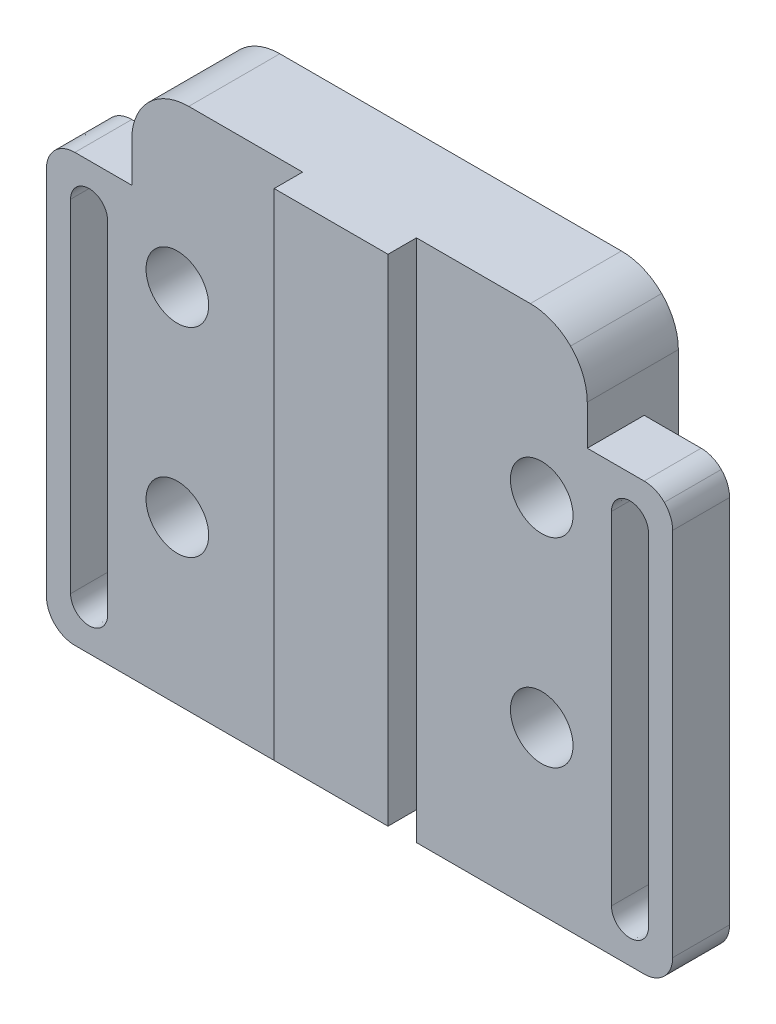
SolidWorks part; units mm, degrees
ref_plane "Front Plane" through (0, 0, 0) normal (0, 0, 1) x (1, 0, 0)
ref_plane "Top Plane" through (0, 0, 0) normal (0, 1, 0) x (1, 0, 0)
ref_plane "Right Plane" through (0, 0, 0) normal (1, 0, 0) x (0, 0, -1)
sketch "Sketch1" plane through (0, 0, 0) normal (0, 0, 1) x (1, 0, 0)
  line L0 (46.2506, -79.8718) -> (46.2506, -72.8718)
  line L1 (-43.7494, -154.8718) -> (56.2506, -154.8718)
  line L2 (-33.7494, -79.8718) -> (-33.7494, -72.8718)
  line L3 (36.2506, -62.8718) -> (-23.7494, -62.8718)
  line L4 (-48.7494, -84.8718) -> (-48.7494, -149.8718)
  line L5 (-33.7494, -79.8718) -> (-43.7494, -79.8718)
  line L6 (-37.9994, -87.3718) -> (-37.9994, -147.3718)
  line L7 (-44.4994, -147.3718) -> (-44.4994, -87.3718)
  line L8 (56.2506, -79.8718) -> (46.2506, -79.8718)
  line L9 (57.0006, -87.3718) -> (57.0006, -147.3718)
  line L10 (50.5006, -147.3718) -> (50.5006, -87.3718)
  line L11 (61.2506, -149.8718) -> (61.2506, -84.8718)
  spline S0 degree 3 poles (43.3217, -65.8007) (43.2437, -65.7242) (43.0879, -65.5713) (42.8451, -65.3519) (42.5959, -65.1403) (42.3398, -64.9371) (42.0768, -64.7421) (41.6283, -64.4317) (40.9724, -64.0382) (40.0838, -63.6184) (39.1583, -63.2868) (38.3634, -63.0881) (37.7184, -62.9759) (37.2313, -62.9161) (36.7418, -62.8787) (36.4145, -62.8741) (36.2506, -62.8718) knots 0 0 0 0 0.041739 0.083393 0.125006 0.166623 0.208289 0.250048 0.374992 0.500007 0.624951 0.749966 0.812537 0.874965 0.937403 1 1 1 1
  spline S1 degree 3 poles (46.2506, -72.8718) (46.2496, -72.7626) (46.2476, -72.5443) (46.231, -72.2174) (46.2044, -71.8916) (46.167, -71.5668) (46.1189, -71.243) (46.0213, -70.7063) (45.8357, -69.9643) (45.5043, -69.0391) (45.0843, -68.1503) (44.6627, -67.4476) (44.286, -66.9122) (43.9838, -66.5255) (43.6641, -66.1529) (43.436, -65.9182) (43.3217, -65.8007) knots 0 0 0 0 0.041739 0.083393 0.125006 0.166623 0.208289 0.250048 0.374992 0.500007 0.624951 0.749966 0.812537 0.874965 0.937403 1 1 1 1
  spline S2 degree 3 poles (-30.8204, -65.8007) (-30.897, -65.8787) (-31.0499, -66.0345) (-31.2692, -66.2774) (-31.4809, -66.5266) (-31.6841, -66.7827) (-31.879, -67.0456) (-32.1894, -67.4942) (-32.5829, -68.1501) (-33.0028, -69.0387) (-33.3344, -69.9641) (-33.5331, -70.7591) (-33.6453, -71.404) (-33.705, -71.8911) (-33.7424, -72.3807) (-33.747, -72.708) (-33.7494, -72.8718) knots 0 0 0 0 0.041739 0.083393 0.125006 0.166623 0.208289 0.250048 0.374992 0.500007 0.624951 0.749966 0.812537 0.874965 0.937403 1 1 1 1
  spline S3 degree 3 poles (-23.7494, -62.8718) (-23.8586, -62.8728) (-24.0769, -62.8749) (-24.4037, -62.8915) (-24.7296, -62.918) (-25.0544, -62.9555) (-25.3782, -63.0035) (-25.9148, -63.1012) (-26.6569, -63.2868) (-27.5821, -63.6182) (-28.4709, -64.0381) (-29.1736, -64.4597) (-29.7089, -64.8365) (-30.0956, -65.1386) (-30.4682, -65.4583) (-30.7029, -65.6865) (-30.8204, -65.8007) knots 0 0 0 0 0.041739 0.083393 0.125006 0.166623 0.208289 0.250048 0.374992 0.500007 0.624951 0.749966 0.812537 0.874965 0.937403 1 1 1 1
  spline S4 degree 3 poles (-25.7494, -94.6218) (-25.6881, -94.6209) (-25.5661, -94.6189) (-25.3842, -94.6032) (-25.2042, -94.5781) (-25.0263, -94.5427) (-24.8503, -94.4972) (-24.6763, -94.4415) (-24.3639, -94.3221) (-23.9314, -94.0925) (-23.437, -93.6845) (-23.0287, -93.1898) (-22.728, -92.6235) (-22.5401, -92.0103) (-22.479, -91.372) (-22.54, -90.7335) (-22.7279, -90.1205) (-23.0286, -89.554) (-23.4368, -89.0595) (-23.9313, -88.6512) (-24.4042, -88.4003) (-24.8047, -88.2562) (-25.114, -88.1788) (-25.4296, -88.1306) (-25.6424, -88.1248) (-25.7494, -88.1218) knots 0 0 0 0 0.018013 0.035886 0.053676 0.07144 0.089234 0.107116 0.125143 0.187594 0.2501 0.312552 0.375058 0.43751 0.500016 0.562468 0.624974 0.687426 0.749932 0.812384 0.87489 0.90631 0.937431 0.968559 1 1 1 1
  spline S5 degree 3 poles (-25.7494, -88.1218) (-25.8106, -88.1228) (-25.9326, -88.1247) (-26.1145, -88.1404) (-26.2945, -88.1655) (-26.4724, -88.201) (-26.6484, -88.2465) (-26.8224, -88.3021) (-27.1348, -88.4216) (-27.5673, -88.6511) (-28.0617, -89.0592) (-28.47, -89.5538) (-28.7707, -90.1201) (-28.9586, -90.7334) (-29.0197, -91.3716) (-28.9587, -92.0101) (-28.7708, -92.6232) (-28.4701, -93.1896) (-28.0619, -93.6842) (-27.5674, -94.0925) (-27.0945, -94.3433) (-26.694, -94.4875) (-26.3847, -94.5648) (-26.0691, -94.613) (-25.8563, -94.6189) (-25.7494, -94.6218) knots 0 0 0 0 0.018013 0.035886 0.053676 0.07144 0.089234 0.107116 0.125143 0.187594 0.2501 0.312552 0.375058 0.43751 0.500016 0.562468 0.624974 0.687426 0.749932 0.812384 0.87489 0.90631 0.937431 0.968559 1 1 1 1
  spline S6 degree 3 poles (-25.7494, -123.1218) (-25.3239, -123.1218) (-24.8987, -123.2064) (-24.1126, -123.532) (-23.7521, -123.7729) (-23.1504, -124.3745) (-22.9095, -124.7351) (-22.5839, -125.5211) (-22.4994, -125.9464) (-22.4994, -126.7972) (-22.5839, -127.2225) (-22.9095, -128.0086) (-23.1504, -128.3691) (-23.7521, -128.9707) (-24.1126, -129.2116) (-24.8987, -129.5372) (-25.3239, -129.6218) (-25.7494, -129.6218) knots 0 0 0 0 0.125 0.125 0.25 0.25 0.375 0.375 0.5 0.5 0.625 0.625 0.75 0.75 0.875 0.875 1 1 1 1
  spline S7 degree 3 poles (-25.7494, -129.6218) (-26.1748, -129.6218) (-26.6, -129.5372) (-27.3861, -129.2116) (-27.7466, -128.9707) (-28.3483, -128.3691) (-28.5892, -128.0086) (-28.9148, -127.2225) (-28.9994, -126.7972) (-28.9994, -125.9464) (-28.9148, -125.5211) (-28.5892, -124.7351) (-28.3483, -124.3745) (-27.7466, -123.7729) (-27.3861, -123.532) (-26.6, -123.2064) (-26.1748, -123.1218) (-25.7494, -123.1218) knots 0 0 0 0 0.125 0.125 0.25 0.25 0.375 0.375 0.5 0.5 0.625 0.625 0.75 0.75 0.875 0.875 1 1 1 1
  spline S8 degree 3 poles (38.2506, -129.6218) (37.8252, -129.6218) (37.4, -129.5372) (36.6139, -129.2116) (36.2534, -128.9707) (35.6517, -128.3691) (35.4108, -128.0086) (35.0852, -127.2225) (35.0006, -126.7972) (35.0006, -125.9464) (35.0852, -125.5211) (35.4108, -124.7351) (35.6517, -124.3745) (36.2534, -123.7729) (36.6139, -123.532) (37.4, -123.2064) (37.8252, -123.1218) (38.2506, -123.1218) knots 0 0 0 0 0.125 0.125 0.25 0.25 0.375 0.375 0.5 0.5 0.625 0.625 0.75 0.75 0.875 0.875 1 1 1 1
  spline S9 degree 3 poles (38.2506, -88.1218) (38.6761, -88.1218) (39.1013, -88.2064) (39.8874, -88.532) (40.2479, -88.7729) (40.8496, -89.3745) (41.0905, -89.7351) (41.4161, -90.5211) (41.5006, -90.9464) (41.5006, -91.7972) (41.4161, -92.2225) (41.0905, -93.0086) (40.8496, -93.3691) (40.2479, -93.9707) (39.8874, -94.2116) (39.1013, -94.5372) (38.6761, -94.6218) (38.2506, -94.6218) knots 0 0 0 0 0.125 0.125 0.25 0.25 0.375 0.375 0.5 0.5 0.625 0.625 0.75 0.75 0.875 0.875 1 1 1 1
  spline S10 degree 3 poles (38.2506, -94.6218) (37.8252, -94.6218) (37.4, -94.5372) (36.6139, -94.2116) (36.2534, -93.9707) (35.6517, -93.3691) (35.4108, -93.0086) (35.0852, -92.2225) (35.0006, -91.7972) (35.0006, -90.9464) (35.0852, -90.5211) (35.4108, -89.7351) (35.6517, -89.3745) (36.2534, -88.7729) (36.6139, -88.532) (37.4, -88.2064) (37.8252, -88.1218) (38.2506, -88.1218) knots 0 0 0 0 0.125 0.125 0.25 0.25 0.375 0.375 0.5 0.5 0.625 0.625 0.75 0.75 0.875 0.875 1 1 1 1
  spline S11 degree 3 poles (38.2506, -123.1218) (38.6761, -123.1218) (39.1013, -123.2064) (39.8874, -123.532) (40.2479, -123.7729) (40.8496, -124.3745) (41.0905, -124.7351) (41.4161, -125.5211) (41.5006, -125.9464) (41.5006, -126.7972) (41.4161, -127.2225) (41.0905, -128.0086) (40.8496, -128.3691) (40.2479, -128.9707) (39.8874, -129.2116) (39.1013, -129.5372) (38.6761, -129.6218) (38.2506, -129.6218) knots 0 0 0 0 0.125 0.125 0.25 0.25 0.375 0.375 0.5 0.5 0.625 0.625 0.75 0.75 0.875 0.875 1 1 1 1
  spline S12 degree 3 poles (-47.2849, -153.4073) (-47.238, -153.4532) (-47.1444, -153.5447) (-46.9974, -153.6748) (-46.8458, -153.7993) (-46.6892, -153.9178) (-46.4476, -154.0862) (-46.1102, -154.2886) (-45.666, -154.4985) (-45.2032, -154.6643) (-44.7793, -154.7704) (-44.4025, -154.8324) (-44.0767, -154.8657) (-43.8586, -154.8698) (-43.7494, -154.8718) knots 0 0 0 0 0.050065 0.100025 0.149957 0.199939 0.250049 0.374961 0.500014 0.624926 0.749979 0.833348 0.916569 1 1 1 1
  spline S13 degree 3 poles (-48.7494, -149.8718) (-48.7486, -149.9373) (-48.7471, -150.0682) (-48.7352, -150.2642) (-48.7161, -150.4594) (-48.6891, -150.654) (-48.6373, -150.9439) (-48.5419, -151.3255) (-48.3762, -151.7881) (-48.1662, -152.2325) (-47.9415, -152.6073) (-47.7189, -152.9176) (-47.512, -153.1716) (-47.3607, -153.3287) (-47.2849, -153.4073) knots 0 0 0 0 0.050065 0.100025 0.149957 0.199939 0.250049 0.374961 0.500014 0.624926 0.749979 0.833348 0.916569 1 1 1 1
  spline S14 degree 3 poles (-47.2849, -81.3363) (-47.3307, -81.3831) (-47.4222, -81.4767) (-47.5523, -81.6238) (-47.6769, -81.7753) (-47.7953, -81.932) (-47.9637, -82.1736) (-48.1661, -82.5109) (-48.3761, -82.9552) (-48.5418, -83.4179) (-48.648, -83.8418) (-48.7099, -84.2186) (-48.7432, -84.5445) (-48.7473, -84.7626) (-48.7494, -84.8718) knots 0 0 0 0 0.050065 0.100025 0.149957 0.199939 0.250049 0.374961 0.500014 0.624926 0.749979 0.833348 0.916569 1 1 1 1
  spline S15 degree 3 poles (-43.7494, -79.8718) (-43.8149, -79.8726) (-43.9458, -79.874) (-44.1417, -79.886) (-44.337, -79.9051) (-44.5315, -79.9321) (-44.8214, -79.9838) (-45.2031, -80.0793) (-45.6657, -80.245) (-46.1101, -80.455) (-46.4849, -80.6797) (-46.7951, -80.9023) (-47.0491, -81.1092) (-47.2062, -81.2605) (-47.2849, -81.3363) knots 0 0 0 0 0.050065 0.100025 0.149957 0.199939 0.250049 0.374961 0.500014 0.624926 0.749979 0.833348 0.916569 1 1 1 1
  spline S16 degree 3 poles (-38.9513, -149.6699) (-38.9895, -149.7071) (-39.0659, -149.7814) (-39.1869, -149.8853) (-39.3123, -149.9834) (-39.4425, -150.075) (-39.5774, -150.1604) (-39.8088, -150.2914) (-40.1503, -150.4433) (-40.6128, -150.5707) (-41.0893, -150.63) (-41.7277, -150.6139) (-42.5113, -150.4185) (-43.2035, -150.0027) (-43.6663, -149.5626) (-43.9612, -149.184) (-44.1982, -148.7667) (-44.3515, -148.3682) (-44.4419, -148.007) (-44.4905, -147.691) (-44.4964, -147.4784) (-44.4994, -147.3718) knots 0 0 0 0 0.020935 0.041773 0.062565 0.08336 0.10421 0.125165 0.187662 0.250231 0.312727 0.375296 0.500018 0.624741 0.687237 0.749806 0.812302 0.874871 0.916632 0.958207 1 1 1 1
  spline S17 degree 3 poles (-37.9994, -147.3718) (-38.0003, -147.4331) (-38.0022, -147.5551) (-38.0179, -147.737) (-38.0431, -147.9169) (-38.0785, -148.0949) (-38.124, -148.2709) (-38.1797, -148.4448) (-38.2615, -148.6587) (-38.3783, -148.907) (-38.5423, -149.1804) (-38.7314, -149.4376) (-38.8777, -149.5922) (-38.9513, -149.6699) knots 0 0 0 0 0.071979 0.1434 0.214488 0.28547 0.356576 0.428033 0.500065 0.625619 0.749978 0.874364 1 1 1 1
  spline S18 degree 3 poles (-38.9513, -85.0737) (-38.9086, -85.1177) (-38.8237, -85.2053) (-38.7062, -85.3451) (-38.5967, -85.4901) (-38.4959, -85.641) (-38.4037, -85.7976) (-38.32, -85.96) (-38.2266, -86.169) (-38.1337, -86.4272) (-38.0564, -86.7365) (-38.0081, -87.0521) (-38.0023, -87.2649) (-37.9994, -87.3718) knots 0 0 0 0 0.071979 0.1434 0.214488 0.28547 0.356576 0.428033 0.500065 0.625619 0.749978 0.874364 1 1 1 1
  spline S19 degree 3 poles (-44.4994, -87.3718) (-44.4986, -87.3184) (-44.4971, -87.212) (-44.485, -87.0528) (-44.4657, -86.8949) (-44.4384, -86.738) (-44.4034, -86.5822) (-44.3324, -86.326) (-44.1983, -85.9771) (-43.9614, -85.5599) (-43.6664, -85.1812) (-43.2036, -84.7411) (-42.5113, -84.3251) (-41.7279, -84.1298) (-41.0894, -84.1136) (-40.6132, -84.1729) (-40.1505, -84.3003) (-39.7603, -84.4737) (-39.4411, -84.6652) (-39.1832, -84.8543) (-39.0287, -85.0005) (-38.9513, -85.0737) knots 0 0 0 0 0.020935 0.041773 0.062565 0.08336 0.10421 0.125165 0.187662 0.250231 0.312727 0.375296 0.500018 0.624741 0.687237 0.749806 0.812302 0.874871 0.916632 0.958207 1 1 1 1
  spline S20 degree 3 poles (59.7862, -81.3363) (59.7393, -81.2905) (59.6457, -81.1989) (59.4987, -81.0688) (59.3471, -80.9443) (59.1905, -80.8258) (58.9489, -80.6574) (58.6115, -80.4551) (58.1673, -80.2451) (57.7045, -80.0794) (57.2806, -79.9732) (56.9038, -79.9112) (56.578, -79.8779) (56.3598, -79.8739) (56.2506, -79.8718) knots 0 0 0 0 0.050065 0.100025 0.149957 0.199939 0.250049 0.374961 0.500014 0.624926 0.749979 0.833348 0.916569 1 1 1 1
  spline S21 degree 3 poles (61.2506, -84.8718) (61.2499, -84.8063) (61.2484, -84.6754) (61.2365, -84.4794) (61.2174, -84.2842) (61.1904, -84.0897) (61.1386, -83.7997) (61.0432, -83.4181) (60.8775, -82.9555) (60.6675, -82.5111) (60.4428, -82.1363) (60.2202, -81.826) (60.0133, -81.5721) (59.862, -81.4149) (59.7862, -81.3363) knots 0 0 0 0 0.050065 0.100025 0.149957 0.199939 0.250049 0.374961 0.500014 0.624926 0.749979 0.833348 0.916569 1 1 1 1
  spline S22 degree 3 poles (56.0487, -85.0737) (56.0914, -85.1177) (56.1763, -85.2053) (56.2938, -85.3451) (56.4033, -85.4901) (56.5041, -85.641) (56.5963, -85.7976) (56.68, -85.96) (56.7734, -86.169) (56.8663, -86.4272) (56.9436, -86.7365) (56.9919, -87.0521) (56.9977, -87.2649) (57.0006, -87.3718) knots 0 0 0 0 0.071979 0.1434 0.214488 0.28547 0.356576 0.428033 0.500065 0.625619 0.749978 0.874364 1 1 1 1
  spline S23 degree 3 poles (50.5006, -87.3718) (50.5014, -87.3184) (50.5029, -87.212) (50.515, -87.0528) (50.5343, -86.8949) (50.5616, -86.738) (50.5966, -86.5822) (50.6676, -86.326) (50.8017, -85.9771) (51.0386, -85.5599) (51.3336, -85.1812) (51.7964, -84.7411) (52.4887, -84.3251) (53.2721, -84.1298) (53.9106, -84.1136) (54.3868, -84.1729) (54.8495, -84.3003) (55.2397, -84.4737) (55.5589, -84.6652) (55.8168, -84.8543) (55.9713, -85.0005) (56.0487, -85.0737) knots 0 0 0 0 0.020935 0.041773 0.062565 0.08336 0.10421 0.125165 0.187662 0.250231 0.312727 0.375296 0.500018 0.624741 0.687237 0.749806 0.812302 0.874871 0.916632 0.958207 1 1 1 1
  spline S24 degree 3 poles (57.0006, -147.3718) (56.9997, -147.4331) (56.9978, -147.5551) (56.9821, -147.737) (56.9569, -147.9169) (56.9215, -148.0949) (56.876, -148.2709) (56.8203, -148.4448) (56.7385, -148.6587) (56.6217, -148.907) (56.4577, -149.1804) (56.2686, -149.4376) (56.1223, -149.5922) (56.0487, -149.6699) knots 0 0 0 0 0.071979 0.1434 0.214488 0.28547 0.356576 0.428033 0.500065 0.625619 0.749978 0.874364 1 1 1 1
  spline S25 degree 3 poles (59.7862, -153.4073) (59.832, -153.3605) (59.9235, -153.2669) (60.0536, -153.1199) (60.1782, -152.9683) (60.2966, -152.8117) (60.465, -152.5701) (60.6674, -152.2327) (60.8774, -151.7885) (61.0431, -151.3257) (61.1492, -150.9018) (61.2112, -150.525) (61.2445, -150.1991) (61.2486, -149.981) (61.2506, -149.8718) knots 0 0 0 0 0.050065 0.100025 0.149957 0.199939 0.250049 0.374961 0.500014 0.624926 0.749979 0.833348 0.916569 1 1 1 1
  spline S26 degree 3 poles (56.0487, -149.6699) (56.0105, -149.7071) (55.9341, -149.7814) (55.8131, -149.8853) (55.6877, -149.9834) (55.5575, -150.075) (55.4226, -150.1604) (55.1912, -150.2914) (54.8497, -150.4433) (54.3872, -150.5707) (53.9107, -150.63) (53.2723, -150.6139) (52.4887, -150.4185) (51.7965, -150.0027) (51.3337, -149.5626) (51.0388, -149.184) (50.8018, -148.7667) (50.6485, -148.3682) (50.5581, -148.007) (50.5095, -147.691) (50.5036, -147.4784) (50.5006, -147.3718) knots 0 0 0 0 0.020935 0.041773 0.062565 0.08336 0.10421 0.125165 0.187662 0.250231 0.312727 0.375296 0.500018 0.624741 0.687237 0.749806 0.812302 0.874871 0.916632 0.958207 1 1 1 1
  spline S27 degree 3 poles (56.2506, -154.8718) (56.3162, -154.8711) (56.4471, -154.8696) (56.643, -154.8576) (56.8383, -154.8385) (57.0328, -154.8116) (57.3227, -154.7598) (57.7044, -154.6643) (58.167, -154.4987) (58.6114, -154.2886) (58.9862, -154.064) (59.2964, -153.8414) (59.5504, -153.6345) (59.7075, -153.4831) (59.7862, -153.4073) knots 0 0 0 0 0.050065 0.100025 0.149957 0.199939 0.250049 0.374961 0.500014 0.624926 0.749979 0.833348 0.916569 1 1 1 1
extrude "Boss-Extrude1" add sketch "Sketch1" along normal blind 16
sketch "Sketch2" plane through (0, 0, 16) normal (0, 0, 1) x (1, 0, 0)
  line L0 (36.2506, -62.8718) -> (-23.7494, -62.8718) construction
  line L1 (16.2506, -149.8718) -> (-3.7494, -149.8718)
  line L2 (16.2506, -149.8718) -> (16.2506, -62.8718)
  line L3 (16.2506, -62.8718) -> (-3.7494, -62.8718)
  line L4 (-3.7494, -149.8718) -> (-3.7494, -62.8718)
  line L5 (16.2506, -149.8718) -> (-3.7494, -62.8718) construction
  line L6 (16.2506, -62.8718) -> (-3.7494, -149.8718) construction
  line L7 (-43.7494, -154.8718) -> (56.2506, -154.8718) construction
  point P0 (6.2506, -106.3718)
  point P9 (6.2506, -62.8718)
  point P13 (6.2506, -154.8718)
  dimension "D1" = 20
  dimension "D2" = 87
extrude "Boss-Extrude2" add sketch "Sketch2" along normal blind 5
sketch "Sketch3" plane through (0, 0, 21) normal (0, 0, 1) x (1, 0, 0)
  line L0 (-3.7494, -149.8718) -> (-3.7494, -154.8718)
  line L1 (-43.7494, -154.8718) -> (56.2506, -154.8718) construction
  line L2 (-3.7494, -154.8718) -> (16.2506, -154.8718)
  line L3 (16.2506, -154.8718) -> (16.2506, -149.8718)
  line L4 (16.2506, -149.8718) -> (-3.7494, -149.8718)
extrude "Cut-Extrude1" cut sketch "Sketch3" against normal blind 11
sketch "Sketch4" plane through (0, 0, 16) normal (0, 0, 1) x (1, 0, 0)
  line L3 (-25.7494, -126.3718) -> (-16.5569, -126.3718) construction
  circle A0 centre (-25.7494, -126.3718) radius 5.5
  circle A1 centre (38.2506, -126.3718) radius 5.5
  circle A2 centre (38.2506, -91.3718) radius 5.5
  circle A3 centre (-25.7494, -91.3718) radius 5.5
  dimension "D1" = 11
  dimension "D2" = 2
  dimension "D3" = 2
extrude "Cut-Extrude2" cut sketch "Sketch4" against normal blind 10
sketch "Sketch5" plane through (0, 0, 0) normal (0, 0, -1) x (-1, 0, 0)
  line L1 (-30.2506, -131.3718) -> (-46.2506, -131.3718)
  line L2 (-30.2506, -131.3718) -> (-30.2506, -86.3718)
  line L3 (-30.2506, -86.3718) -> (-46.2506, -86.3718)
  line L4 (-46.2506, -131.3718) -> (-46.2506, -86.3718)
  line L5 (-30.2506, -131.3718) -> (-46.2506, -86.3718) construction
  line L6 (-30.2506, -86.3718) -> (-46.2506, -131.3718) construction
  line L9 (-46.2506, -79.8718) -> (-46.2506, -72.8718) construction
  line L10 (-6.2506, -62.8718) -> (-6.2506, -73.4746) construction
  line L11 (-36.2506, -62.8718) -> (23.7494, -62.8718) construction
  line L12 (17.7494, -86.3718) -> (33.7494, -131.3718) construction
  line L13 (17.7494, -131.3718) -> (33.7494, -86.3718) construction
  line L16 (33.7494, -131.3718) -> (33.7494, -86.3718)
  line L17 (17.7494, -86.3718) -> (33.7494, -86.3718)
  line L18 (17.7494, -131.3718) -> (17.7494, -86.3718)
  line L19 (17.7494, -131.3718) -> (33.7494, -131.3718)
  point P0 (-38.2506, -108.8718)
  point P25 (25.7494, -108.8718)
  dimension "D1" = 16
  dimension "D2" = 45
extrude "Cut-Extrude3" cut sketch "Sketch5" against normal blind 1
sketch "Sketch6" plane through (0, 0, 0) normal (0, 0, -1) x (-1, 0, 0)
  line L0 (-46.2506, -79.8718) -> (-46.2506, -154.8718)
  line L1 (43.7494, -154.8718) -> (-56.2506, -154.8718) construction
  line L2 (-57.0006, -147.3718) -> (-57.0006, -87.3718) construction
  line L3 (-57.0006, -147.3718) -> (-57.0006, -87.3718)
  line L4 (-50.5006, -87.3718) -> (-50.5006, -147.3718) construction
  line L5 (-50.5006, -87.3718) -> (-50.5006, -147.3718)
  line L6 (-46.2506, -154.8718) -> (-56.2506, -154.8718)
  line L7 (-6.2506, -154.8718) -> (-6.2506, -140.574) construction
  line L10 (-46.2506, -72.8718) -> (-46.2506, -79.8718)
  line L11 (-46.2506, -79.8718) -> (-56.2506, -79.8718)
  line L12 (-61.2506, -84.8718) -> (-61.2506, -149.8718)
  line L13 (-56.2506, -154.8718) -> (43.7494, -154.8718)
  line L14 (48.7494, -149.8718) -> (48.7494, -84.8718)
  line L15 (43.7494, -79.8718) -> (33.7494, -79.8718)
  line L16 (33.7494, -79.8718) -> (33.7494, -72.8718)
  line L17 (23.7494, -62.8718) -> (-36.2506, -62.8718)
  line L19 (-46.2506, -79.8718) -> (-56.2506, -79.8718)
  line L20 (-61.2506, -84.8718) -> (-61.2506, -149.8718)
  line L30 (33.7494, -79.8718) -> (33.7494, -154.8718)
  line L31 (33.7494, -154.8718) -> (43.7494, -154.8718)
  line L32 (33.7494, -79.8718) -> (43.7494, -79.8718)
  line L33 (48.7494, -84.8718) -> (48.7494, -149.8718) construction
  line L34 (48.7494, -84.8718) -> (48.7494, -149.8718)
  line L35 (44.4994, -87.3718) -> (44.4994, -147.3718) construction
  line L36 (37.9994, -147.3718) -> (37.9994, -87.3718) construction
  line L37 (44.4994, -87.3718) -> (44.4994, -147.3718)
  line L38 (37.9994, -147.3718) -> (37.9994, -87.3718)
  spline S0 degree 3 poles (-2027.4066, 2176.0249) (-42.345, -125.957) (-62.4154, -89.6938) (-55.5589, -84.6652) (-55.2397, -84.4737) (-54.8495, -84.3003) (-54.3868, -84.1729) (-53.9106, -84.1136) (-53.2721, -84.1298) (-52.4887, -84.3251) (-51.7964, -84.7411) (-51.3336, -85.1812) (-51.0386, -85.5599) (-50.8017, -85.9771) (-50.6676, -86.326) (-50.5966, -86.5822) (-50.5616, -86.738) (-50.5343, -86.8949) (-50.515, -87.0528) (-50.0095, -93.701) (-74.9187, -101.2707) (2947.83, 8.0716) knots -3.202284 -3.202284 -3.202284 -3.202284 0.041793 0.083368 0.125129 0.187698 0.250194 0.312763 0.375259 0.499982 0.624704 0.687273 0.749769 0.812338 0.874835 0.89579 0.91664 0.937435 0.958227 0.979065 3.551551 3.551551 3.551551 3.551551 only from (-56.0487, -85.0737) to (-50.5006, -87.3718) construction
  spline S1 degree 3 poles (-56.0487, -85.0737) (-55.9713, -85.0005) (-55.8168, -84.8543) (-55.5589, -84.6652) (-55.2397, -84.4737) (-54.8495, -84.3003) (-54.3868, -84.1729) (-53.9106, -84.1136) (-53.2721, -84.1298) (-52.4887, -84.3251) (-51.7964, -84.7411) (-51.3336, -85.1812) (-51.0386, -85.5599) (-50.8017, -85.9771) (-50.6676, -86.326) (-50.5966, -86.5822) (-50.5616, -86.738) (-50.5343, -86.8949) (-50.515, -87.0528) (-50.5029, -87.212) (-50.5014, -87.3184) (-50.5006, -87.3718) knots 0 0 0 0 0.041793 0.083368 0.125129 0.187698 0.250194 0.312763 0.375259 0.499982 0.624704 0.687273 0.749769 0.812338 0.874835 0.89579 0.91664 0.937435 0.958227 0.979065 1 1 1 1
  spline S2 degree 3 poles (-3049.9078, 116.4435) (-18.3774, -106.6249) (-58.2318, -95.1636) (-56.9436, -86.7365) (-56.8663, -86.4272) (-56.7734, -86.169) (-56.68, -85.96) (-56.5963, -85.7976) (-56.5041, -85.641) (-56.4033, -85.4901) (-56.2938, -85.3451) (-51.7772, -79.9754) (-26.7535, -93.4896) (-2253.3466, 1957.3042) knots -9.622076 -9.622076 -9.622076 -9.622076 0.125636 0.250022 0.374381 0.499935 0.571967 0.643424 0.71453 0.785512 0.8566 0.928021 9.027047 9.027047 9.027047 9.027047 only from (-57.0006, -87.3718) to (-56.0487, -85.0737) construction
  spline S3 degree 3 poles (-57.0006, -87.3718) (-56.9977, -87.2649) (-56.9919, -87.0521) (-56.9436, -86.7365) (-56.8663, -86.4272) (-56.7734, -86.169) (-56.68, -85.96) (-56.5963, -85.7976) (-56.5041, -85.641) (-56.4033, -85.4901) (-56.2938, -85.3451) (-56.1763, -85.2053) (-56.0914, -85.1177) (-56.0487, -85.0737) knots 0 0 0 0 0.125636 0.250022 0.374381 0.499935 0.571967 0.643424 0.71453 0.785512 0.8566 0.928021 1 1 1 1
  spline S4 degree 3 poles (2942.298, -352.2494) (-89.0995, -128.1529) (-49.2656, -139.603) (-50.5581, -148.007) (-50.6485, -148.3682) (-50.8018, -148.7667) (-51.0388, -149.184) (-51.3337, -149.5626) (-51.7965, -150.0027) (-52.4887, -150.4185) (-53.2723, -150.6139) (-53.9107, -150.63) (-54.3872, -150.5707) (-54.8497, -150.4433) (-55.1912, -150.2914) (-55.4226, -150.1604) (-55.5575, -150.075) (-55.6877, -149.9834) (-55.8131, -149.8853) (-60.8715, -145.5418) (-48.6106, -122.5757) (-2108.7, -2337.2985) knots -3.202284 -3.202284 -3.202284 -3.202284 0.041793 0.083368 0.125129 0.187698 0.250194 0.312763 0.375259 0.499982 0.624704 0.687273 0.749769 0.812338 0.874835 0.89579 0.91664 0.937435 0.958227 0.979065 3.551551 3.551551 3.551551 3.551551 only from (-50.5006, -147.3718) to (-56.0487, -149.6699) construction
  spline S5 degree 3 poles (-50.5006, -147.3718) (-50.5036, -147.4784) (-50.5095, -147.691) (-50.5581, -148.007) (-50.6485, -148.3682) (-50.8018, -148.7667) (-51.0388, -149.184) (-51.3337, -149.5626) (-51.7965, -150.0027) (-52.4887, -150.4185) (-53.2723, -150.6139) (-53.9107, -150.63) (-54.3872, -150.5707) (-54.8497, -150.4433) (-55.1912, -150.2914) (-55.4226, -150.1604) (-55.5575, -150.075) (-55.6877, -149.9834) (-55.8131, -149.8853) (-55.9341, -149.7814) (-56.0105, -149.7071) (-56.0487, -149.6699) knots 0 0 0 0 0.041793 0.083368 0.125129 0.187698 0.250194 0.312763 0.375259 0.499982 0.624704 0.687273 0.749769 0.812338 0.874835 0.89579 0.91664 0.937435 0.958227 0.979065 1 1 1 1
  spline S6 degree 3 poles (-2316.4728, -2121.8557) (-15.124, -135.9732) (-51.4096, -156.0501) (-56.4577, -149.1804) (-56.6217, -148.907) (-56.7385, -148.6587) (-56.8203, -148.4448) (-56.876, -148.2709) (-56.9215, -148.0949) (-56.9569, -147.9169) (-56.9821, -147.737) (-57.5853, -140.7463) (-30.3348, -132.6079) (-3054.9041, -256.9167) knots -9.622076 -9.622076 -9.622076 -9.622076 0.125636 0.250022 0.374381 0.499935 0.571967 0.643424 0.71453 0.785512 0.8566 0.928021 9.027047 9.027047 9.027047 9.027047 only from (-56.0487, -149.6699) to (-57.0006, -147.3718) construction
  spline S7 degree 3 poles (-56.0487, -149.6699) (-56.1223, -149.5922) (-56.2686, -149.4376) (-56.4577, -149.1804) (-56.6217, -148.907) (-56.7385, -148.6587) (-56.8203, -148.4448) (-56.876, -148.2709) (-56.9215, -148.0949) (-56.9569, -147.9169) (-56.9821, -147.737) (-56.9978, -147.5551) (-56.9997, -147.4331) (-57.0006, -147.3718) knots 0 0 0 0 0.125636 0.250022 0.374381 0.499935 0.571967 0.643424 0.71453 0.785512 0.8566 0.928021 1 1 1 1
  spline S8 degree 3 poles (2216.2512, 1990.9412) (18.2653, -86.6751) (42.1004, -75.4628) (47.5523, -81.6238) (47.6769, -81.7753) (47.7953, -81.932) (47.9637, -82.1736) (48.1661, -82.5109) (48.3761, -82.9552) (48.5418, -83.4179) (48.648, -83.8418) (48.7099, -84.2186) (49.7106, -94.015) (14.6956, -105.5474) (3046.0394, 40.1273) knots -6.134029 -6.134029 -6.134029 -6.134029 0.050065 0.100025 0.149957 0.199939 0.250049 0.374961 0.500014 0.624926 0.749979 0.833348 0.916569 8.266403 8.266403 8.266403 8.266403 only from (47.2849, -81.3363) to (48.7494, -84.8718) construction
  spline S9 degree 3 poles (112.1187, 2919.1404) (27.0045, -104.1669) (35.9302, -79.3846) (44.1417, -79.886) (44.337, -79.9051) (44.5315, -79.9321) (44.8214, -79.9838) (45.2031, -80.0793) (45.6657, -80.245) (46.1101, -80.455) (46.4849, -80.6797) (46.7951, -80.9023) (54.4298, -87.1218) (37.8251, -120.0358) (2078.3013, 2126.4556) knots -6.134029 -6.134029 -6.134029 -6.134029 0.050065 0.100025 0.149957 0.199939 0.250049 0.374961 0.500014 0.624926 0.749979 0.833348 0.916569 8.266403 8.266403 8.266403 8.266403 only from (43.7494, -79.8718) to (47.2849, -81.3363) construction
  spline S10 degree 3 poles (47.2849, -81.3363) (47.3307, -81.3831) (47.4222, -81.4767) (47.5523, -81.6238) (47.6769, -81.7753) (47.7953, -81.932) (47.9637, -82.1736) (48.1661, -82.5109) (48.3761, -82.9552) (48.5418, -83.4179) (48.648, -83.8418) (48.7099, -84.2186) (48.7432, -84.5445) (48.7473, -84.7626) (48.7494, -84.8718) knots 0 0 0 0 0.050065 0.100025 0.149957 0.199939 0.250049 0.374961 0.500014 0.624926 0.749979 0.833348 0.916569 1 1 1 1
  spline S11 degree 3 poles (43.7494, -79.8718) (43.8149, -79.8726) (43.9458, -79.874) (44.1417, -79.886) (44.337, -79.9051) (44.5315, -79.9321) (44.8214, -79.9838) (45.2031, -80.0793) (45.6657, -80.245) (46.1101, -80.455) (46.4849, -80.6797) (46.7951, -80.9023) (47.0491, -81.1092) (47.2062, -81.2605) (47.2849, -81.3363) knots 0 0 0 0 0.050065 0.100025 0.149957 0.199939 0.250049 0.374961 0.500014 0.624926 0.749979 0.833348 0.916569 1 1 1 1
  spline S12 degree 3 poles (-757.5456, 634.1163) (-17.5261, -63.9657) (-37.4631, -58.9259) (-43.9838, -66.5255) (-44.286, -66.9122) (-44.6627, -67.4476) (-45.0843, -68.1503) (-45.5043, -69.0391) (-45.8357, -69.9643) (-46.0213, -70.7063) (-46.1189, -71.243) (-46.167, -71.5668) (-46.2044, -71.8916) (-46.231, -72.2174) (-46.67, -80.8554) (-33.2776, -89.74) (-1046.2275, -72.1326) knots -3.636061 -3.636061 -3.636061 -3.636061 0.062597 0.125035 0.187463 0.250034 0.375049 0.499993 0.625008 0.749952 0.791711 0.833377 0.874994 0.916607 0.958261 4.178587 4.178587 4.178587 4.178587 only from (-43.3217, -65.8007) to (-46.2506, -72.8718)
  spline S13 degree 3 poles (-229.5417, 3916.1076) (-33.2886, -121.1621) (-46.1546, -78.8133) (-56.9038, -79.9112) (-57.2806, -79.9732) (-57.7045, -80.0794) (-58.1673, -80.2451) (-58.6115, -80.4551) (-58.9489, -80.6574) (-59.1905, -80.8258) (-59.3471, -80.9443) (-59.4987, -81.0688) (-66.2649, -87.0563) (-52.0569, -115.2571) (-2818.7869, 2814.5065) knots -7.997523 -7.997523 -7.997523 -7.997523 0.083431 0.166652 0.250021 0.375074 0.499986 0.625039 0.749951 0.800061 0.850043 0.899975 0.949935 7.751349 7.751349 7.751349 7.751349 only from (-56.2506, -79.8718) to (-59.7862, -81.3363)
  spline S14 degree 3 poles (-3007.9055, 2621.7126) (-14.3529, -94.2963) (-53.3957, -73.4488) (-60.2202, -81.826) (-60.4428, -82.1363) (-60.6675, -82.5111) (-60.8775, -82.9555) (-61.0432, -83.4181) (-61.1386, -83.7997) (-61.1904, -84.0897) (-61.2174, -84.2842) (-61.2365, -84.4794) (-61.7872, -93.4977) (-31.7996, -103.392) (-4059.8288, 11.8901) knots -7.997523 -7.997523 -7.997523 -7.997523 0.083431 0.166652 0.250021 0.375074 0.499986 0.625039 0.749951 0.800061 0.850043 0.899975 0.949935 7.751349 7.751349 7.751349 7.751349 only from (-59.7862, -81.3363) to (-61.2506, -84.8718)
  spline S15 degree 3 poles (-4057.23, -323.1628) (-19.9604, -126.9098) (-62.3092, -139.7757) (-61.2112, -150.525) (-61.1492, -150.9018) (-61.0431, -151.3257) (-60.8774, -151.7885) (-60.6674, -152.2327) (-60.465, -152.5701) (-60.2966, -152.8117) (-60.1782, -152.9683) (-60.0536, -153.1199) (-54.0662, -159.8861) (-25.8654, -145.6781) (-2955.6289, -2912.4081) knots -7.997523 -7.997523 -7.997523 -7.997523 0.083431 0.166652 0.250021 0.375074 0.499986 0.625039 0.749951 0.800061 0.850043 0.899975 0.949935 7.751349 7.751349 7.751349 7.751349 only from (-61.2506, -149.8718) to (-59.7862, -153.4073)
  spline S16 degree 3 poles (-2762.835, -3101.5267) (-46.8262, -107.9741) (-67.6737, -147.0168) (-59.2964, -153.8414) (-58.9862, -154.064) (-58.6114, -154.2886) (-58.167, -154.4987) (-57.7044, -154.6643) (-57.3227, -154.7598) (-57.0328, -154.8116) (-56.8383, -154.8385) (-56.643, -154.8576) (-47.6248, -155.4083) (-37.7304, -125.4208) (-153.0126, -4153.45) knots -7.997523 -7.997523 -7.997523 -7.997523 0.083431 0.166652 0.250021 0.375074 0.499986 0.625039 0.749951 0.800061 0.850043 0.899975 0.949935 7.751349 7.751349 7.751349 7.751349 only from (-59.7862, -153.4073) to (-56.2506, -154.8718)
  spline S17 degree 3 poles (75.1528, -1154.378) (29.8209, -138.5728) (37.5097, -155.5365) (44.4025, -154.8324) (44.7793, -154.7704) (45.2032, -154.6643) (45.666, -154.4985) (46.1102, -154.2886) (46.4476, -154.0862) (46.6892, -153.9178) (46.8458, -153.7993) (46.9974, -153.6748) (51.3145, -149.8546) (47.1346, -137.0923) (744.3308, -870.425) knots -5.038607 -5.038607 -5.038607 -5.038607 0.083431 0.166652 0.250021 0.375074 0.499986 0.625039 0.749951 0.800061 0.850043 0.899975 0.949935 5.253276 5.253276 5.253276 5.253276 only from (43.7494, -154.8718) to (47.2849, -153.4073)
  spline S18 degree 3 poles (776.2481, -837.9594) (25.9109, -151.7311) (43.3428, -158.2894) (47.7189, -152.9176) (47.9415, -152.6073) (48.1662, -152.2325) (48.3762, -151.7881) (48.5419, -151.3255) (48.6373, -150.9439) (48.6891, -150.654) (48.7161, -150.4594) (48.7352, -150.2642) (49.0865, -144.5103) (37.1066, -138.4416) (1048.6432, -163.994) knots -5.038607 -5.038607 -5.038607 -5.038607 0.083431 0.166652 0.250021 0.375074 0.499986 0.625039 0.749951 0.800061 0.850043 0.899975 0.949935 5.253276 5.253276 5.253276 5.253276 only from (47.2849, -153.4073) to (48.7494, -149.8718)
  spline S19 degree 3 poles (1048.2555, -53.4684) (32.4504, -98.8002) (49.414, -91.1115) (48.7099, -84.2186) (48.648, -83.8418) (48.5418, -83.4179) (48.3761, -82.9552) (48.1661, -82.5109) (47.9637, -82.1736) (47.7953, -81.932) (47.6769, -81.7753) (47.5523, -81.6238) (43.7322, -77.3067) (30.9698, -81.4866) (764.3025, 615.7096) knots -5.038607 -5.038607 -5.038607 -5.038607 0.083431 0.166652 0.250021 0.375074 0.499986 0.625039 0.749951 0.800061 0.850043 0.899975 0.949935 5.253276 5.253276 5.253276 5.253276 only from (48.7494, -84.8718) to (47.2849, -81.3363)
  spline S20 degree 3 poles (731.8369, 647.6269) (45.6086, -102.7103) (52.167, -85.2784) (46.7951, -80.9023) (46.4849, -80.6797) (46.1101, -80.455) (45.6657, -80.245) (45.2031, -80.0793) (44.8214, -79.9838) (44.5315, -79.9321) (44.337, -79.9051) (44.1417, -79.886) (38.3879, -79.5346) (32.3192, -91.5146) (57.8715, 920.0221) knots -5.038607 -5.038607 -5.038607 -5.038607 0.083431 0.166652 0.250021 0.375074 0.499986 0.625039 0.749951 0.800061 0.850043 0.899975 0.949935 5.253276 5.253276 5.253276 5.253276 only from (47.2849, -81.3363) to (43.7494, -79.8718)
  spline S21 degree 3 poles (1033.698, -62.7553) (16.8067, -92.4096) (34.468, -81.8757) (33.705, -71.8911) (33.6453, -71.404) (33.5331, -70.7591) (33.3344, -69.9641) (33.0028, -69.0387) (32.5829, -68.1501) (32.1894, -67.4942) (31.879, -67.0456) (31.6841, -66.7827) (31.4809, -66.5266) (31.2692, -66.2774) (25.4717, -59.859) (9.7195, -63.0465) (738.4335, 640.7669) knots -3.636061 -3.636061 -3.636061 -3.636061 0.062597 0.125035 0.187463 0.250034 0.375049 0.499993 0.625008 0.749952 0.791711 0.833377 0.874994 0.916607 0.958261 4.178587 4.178587 4.178587 4.178587 only from (33.7494, -72.8718) to (30.8204, -65.8007)
  spline S22 degree 3 poles (730.7375, 648.4231) (32.6555, -91.5963) (37.6953, -71.6593) (30.0956, -65.1386) (29.7089, -64.8365) (29.1736, -64.4597) (28.4709, -64.0381) (27.5821, -63.6182) (26.6569, -63.2868) (25.9148, -63.1012) (25.3782, -63.0035) (25.0544, -62.9555) (24.7296, -62.918) (24.4037, -62.8915) (15.7658, -62.4524) (6.8812, -75.8449) (24.4886, 937.105) knots -3.636061 -3.636061 -3.636061 -3.636061 0.062597 0.125035 0.187463 0.250034 0.375049 0.499993 0.625008 0.749952 0.791711 0.833377 0.874994 0.916607 0.958261 4.178587 4.178587 4.178587 4.178587 only from (30.8204, -65.8007) to (23.7494, -62.8718)
  spline S23 degree 3 poles (-46.3671, 937.0768) (-16.7128, -79.8145) (-27.2467, -62.1532) (-37.2313, -62.9161) (-37.7184, -62.9759) (-38.3634, -63.0881) (-39.1583, -63.2868) (-40.0838, -63.6184) (-40.9724, -64.0382) (-41.6283, -64.4317) (-42.0768, -64.7421) (-42.3398, -64.9371) (-42.5959, -65.1403) (-42.8451, -65.3519) (-49.2635, -71.1494) (-46.076, -86.9017) (-749.8894, 641.8124) knots -3.636061 -3.636061 -3.636061 -3.636061 0.062597 0.125035 0.187463 0.250034 0.375049 0.499993 0.625008 0.749952 0.791711 0.833377 0.874994 0.916607 0.958261 4.178587 4.178587 4.178587 4.178587 only from (-36.2506, -62.8718) to (-43.3217, -65.8007)
  spline S24 degree 3 poles (-2221.4728, -2121.8557) (79.876, -135.9732) (43.5904, -156.0501) (38.5423, -149.1804) (38.3783, -148.907) (38.2615, -148.6587) (38.1797, -148.4448) (38.124, -148.2709) (38.0785, -148.0949) (38.0431, -147.9169) (38.0179, -147.737) (37.4147, -140.7463) (64.6652, -132.6079) (-2959.9041, -256.9167) knots -9.622076 -9.622076 -9.622076 -9.622076 0.125636 0.250022 0.374381 0.499935 0.571967 0.643424 0.71453 0.785512 0.8566 0.928021 9.027047 9.027047 9.027047 9.027047 only from (38.9513, -149.6699) to (37.9994, -147.3718) construction
  spline S25 degree 3 poles (-56.2506, -79.8718) (-56.3598, -79.8739) (-56.578, -79.8779) (-56.9038, -79.9112) (-57.2806, -79.9732) (-57.7045, -80.0794) (-58.1673, -80.2451) (-58.6115, -80.4551) (-58.9489, -80.6574) (-59.1905, -80.8258) (-59.3471, -80.9443) (-59.4987, -81.0688) (-59.6457, -81.1989) (-59.7393, -81.2905) (-59.7862, -81.3363) knots 0 0 0 0 0.083431 0.166652 0.250021 0.375074 0.499986 0.625039 0.749951 0.800061 0.850043 0.899975 0.949935 1 1 1 1
  spline S26 degree 3 poles (-59.7862, -81.3363) (-59.862, -81.4149) (-60.0133, -81.5721) (-60.2202, -81.826) (-60.4428, -82.1363) (-60.6675, -82.5111) (-60.8775, -82.9555) (-61.0432, -83.4181) (-61.1386, -83.7997) (-61.1904, -84.0897) (-61.2174, -84.2842) (-61.2365, -84.4794) (-61.2484, -84.6754) (-61.2499, -84.8063) (-61.2506, -84.8718) knots 0 0 0 0 0.083431 0.166652 0.250021 0.375074 0.499986 0.625039 0.749951 0.800061 0.850043 0.899975 0.949935 1 1 1 1
  spline S27 degree 3 poles (-61.2506, -149.8718) (-61.2486, -149.981) (-61.2445, -150.1991) (-61.2112, -150.525) (-61.1492, -150.9018) (-61.0431, -151.3257) (-60.8774, -151.7885) (-60.6674, -152.2327) (-60.465, -152.5701) (-60.2966, -152.8117) (-60.1782, -152.9683) (-60.0536, -153.1199) (-59.9235, -153.2669) (-59.832, -153.3605) (-59.7862, -153.4073) knots 0 0 0 0 0.083431 0.166652 0.250021 0.375074 0.499986 0.625039 0.749951 0.800061 0.850043 0.899975 0.949935 1 1 1 1
  spline S28 degree 3 poles (-59.7862, -153.4073) (-59.7075, -153.4831) (-59.5504, -153.6345) (-59.2964, -153.8414) (-58.9862, -154.064) (-58.6114, -154.2886) (-58.167, -154.4987) (-57.7044, -154.6643) (-57.3227, -154.7598) (-57.0328, -154.8116) (-56.8383, -154.8385) (-56.643, -154.8576) (-56.4471, -154.8696) (-56.3162, -154.8711) (-56.2506, -154.8718) knots 0 0 0 0 0.083431 0.166652 0.250021 0.375074 0.499986 0.625039 0.749951 0.800061 0.850043 0.899975 0.949935 1 1 1 1
  spline S29 degree 3 poles (3037.298, -352.2494) (5.9005, -128.1529) (45.7344, -139.603) (44.4419, -148.007) (44.3515, -148.3682) (44.1982, -148.7667) (43.9612, -149.184) (43.6663, -149.5626) (43.2035, -150.0027) (42.5113, -150.4185) (41.7277, -150.6139) (41.0893, -150.63) (40.6128, -150.5707) (40.1503, -150.4433) (39.8088, -150.2914) (39.5774, -150.1604) (39.4425, -150.075) (39.3123, -149.9834) (39.1869, -149.8853) (34.1285, -145.5418) (46.3894, -122.5757) (-2013.7, -2337.2985) knots -3.202284 -3.202284 -3.202284 -3.202284 0.041793 0.083368 0.125129 0.187698 0.250194 0.312763 0.375259 0.499982 0.624704 0.687273 0.749769 0.812338 0.874835 0.89579 0.91664 0.937435 0.958227 0.979065 3.551551 3.551551 3.551551 3.551551 only from (44.4994, -147.3718) to (38.9513, -149.6699) construction
  spline S30 degree 3 poles (2119.5624, -2322.3736) (41.9461, -124.3877) (53.1584, -148.2229) (46.9974, -153.6748) (46.8458, -153.7993) (46.6892, -153.9178) (46.4476, -154.0862) (46.1102, -154.2886) (45.666, -154.4985) (45.2032, -154.6643) (44.7793, -154.7704) (44.4025, -154.8324) (34.6062, -155.833) (23.0738, -120.8181) (168.7484, -3152.1619) knots -6.134029 -6.134029 -6.134029 -6.134029 0.050065 0.100025 0.149957 0.199939 0.250049 0.374961 0.500014 0.624926 0.749979 0.833348 0.916569 8.266403 8.266403 8.266403 8.266403 only from (47.2849, -153.4073) to (43.7494, -154.8718) construction
  spline S31 degree 3 poles (3047.7616, -218.2411) (24.4543, -133.127) (49.2366, -142.0527) (48.7352, -150.2642) (48.7161, -150.4594) (48.6891, -150.654) (48.6373, -150.9439) (48.5419, -151.3255) (48.3762, -151.7881) (48.1662, -152.2325) (47.9415, -152.6073) (47.7189, -152.9176) (41.4994, -160.5523) (8.5854, -143.9475) (2255.0767, -2184.4238) knots -6.134029 -6.134029 -6.134029 -6.134029 0.050065 0.100025 0.149957 0.199939 0.250049 0.374961 0.500014 0.624926 0.749979 0.833348 0.916569 8.266403 8.266403 8.266403 8.266403 only from (48.7494, -149.8718) to (47.2849, -153.4073) construction
  spline S32 degree 3 poles (38.9513, -149.6699) (38.8777, -149.5922) (38.7314, -149.4376) (38.5423, -149.1804) (38.3783, -148.907) (38.2615, -148.6587) (38.1797, -148.4448) (38.124, -148.2709) (38.0785, -148.0949) (38.0431, -147.9169) (38.0179, -147.737) (38.0022, -147.5551) (38.0003, -147.4331) (37.9994, -147.3718) knots 0 0 0 0 0.125636 0.250022 0.374381 0.499935 0.571967 0.643424 0.71453 0.785512 0.8566 0.928021 1 1 1 1
  spline S33 degree 3 poles (44.4994, -147.3718) (44.4964, -147.4784) (44.4905, -147.691) (44.4419, -148.007) (44.3515, -148.3682) (44.1982, -148.7667) (43.9612, -149.184) (43.6663, -149.5626) (43.2035, -150.0027) (42.5113, -150.4185) (41.7277, -150.6139) (41.0893, -150.63) (40.6128, -150.5707) (40.1503, -150.4433) (39.8088, -150.2914) (39.5774, -150.1604) (39.4425, -150.075) (39.3123, -149.9834) (39.1869, -149.8853) (39.0659, -149.7814) (38.9895, -149.7071) (38.9513, -149.6699) knots 0 0 0 0 0.041793 0.083368 0.125129 0.187698 0.250194 0.312763 0.375259 0.499982 0.624704 0.687273 0.749769 0.812338 0.874835 0.89579 0.91664 0.937435 0.958227 0.979065 1 1 1 1
  spline S34 degree 3 poles (47.2849, -153.4073) (47.238, -153.4532) (47.1444, -153.5447) (46.9974, -153.6748) (46.8458, -153.7993) (46.6892, -153.9178) (46.4476, -154.0862) (46.1102, -154.2886) (45.666, -154.4985) (45.2032, -154.6643) (44.7793, -154.7704) (44.4025, -154.8324) (44.0767, -154.8657) (43.8586, -154.8698) (43.7494, -154.8718) knots 0 0 0 0 0.050065 0.100025 0.149957 0.199939 0.250049 0.374961 0.500014 0.624926 0.749979 0.833348 0.916569 1 1 1 1
  spline S35 degree 3 poles (48.7494, -149.8718) (48.7486, -149.9373) (48.7471, -150.0682) (48.7352, -150.2642) (48.7161, -150.4594) (48.6891, -150.654) (48.6373, -150.9439) (48.5419, -151.3255) (48.3762, -151.7881) (48.1662, -152.2325) (47.9415, -152.6073) (47.7189, -152.9176) (47.512, -153.1716) (47.3607, -153.3287) (47.2849, -153.4073) knots 0 0 0 0 0.050065 0.100025 0.149957 0.199939 0.250049 0.374961 0.500014 0.624926 0.749979 0.833348 0.916569 1 1 1 1
  spline S36 degree 3 poles (-1932.4066, 2176.0249) (52.655, -125.957) (32.5846, -89.6938) (39.4411, -84.6652) (39.7603, -84.4737) (40.1505, -84.3003) (40.6132, -84.1729) (41.0894, -84.1136) (41.7279, -84.1298) (42.5113, -84.3251) (43.2036, -84.7411) (43.6664, -85.1812) (43.9614, -85.5599) (44.1983, -85.9771) (44.3324, -86.326) (44.4034, -86.5822) (44.4384, -86.738) (44.4657, -86.8949) (44.485, -87.0528) (44.9905, -93.701) (20.0813, -101.2707) (3042.83, 8.0716) knots -3.202284 -3.202284 -3.202284 -3.202284 0.041793 0.083368 0.125129 0.187698 0.250194 0.312763 0.375259 0.499982 0.624704 0.687273 0.749769 0.812338 0.874835 0.89579 0.91664 0.937435 0.958227 0.979065 3.551551 3.551551 3.551551 3.551551 only from (38.9513, -85.0737) to (44.4994, -87.3718) construction
  spline S37 degree 3 poles (-2954.9078, 116.4435) (76.6226, -106.6249) (36.7682, -95.1636) (38.0564, -86.7365) (38.1337, -86.4272) (38.2266, -86.169) (38.32, -85.96) (38.4037, -85.7976) (38.4959, -85.641) (38.5967, -85.4901) (38.7062, -85.3451) (43.2228, -79.9754) (68.2465, -93.4896) (-2158.3466, 1957.3042) knots -9.622076 -9.622076 -9.622076 -9.622076 0.125636 0.250022 0.374381 0.499935 0.571967 0.643424 0.71453 0.785512 0.8566 0.928021 9.027047 9.027047 9.027047 9.027047 only from (37.9994, -87.3718) to (38.9513, -85.0737) construction
  spline S38 degree 3 poles (38.9513, -85.0737) (39.0287, -85.0005) (39.1832, -84.8543) (39.4411, -84.6652) (39.7603, -84.4737) (40.1505, -84.3003) (40.6132, -84.1729) (41.0894, -84.1136) (41.7279, -84.1298) (42.5113, -84.3251) (43.2036, -84.7411) (43.6664, -85.1812) (43.9614, -85.5599) (44.1983, -85.9771) (44.3324, -86.326) (44.4034, -86.5822) (44.4384, -86.738) (44.4657, -86.8949) (44.485, -87.0528) (44.4971, -87.212) (44.4986, -87.3184) (44.4994, -87.3718) knots 0 0 0 0 0.041793 0.083368 0.125129 0.187698 0.250194 0.312763 0.375259 0.499982 0.624704 0.687273 0.749769 0.812338 0.874835 0.89579 0.91664 0.937435 0.958227 0.979065 1 1 1 1
  spline S39 degree 3 poles (37.9994, -87.3718) (38.0023, -87.2649) (38.0081, -87.0521) (38.0564, -86.7365) (38.1337, -86.4272) (38.2266, -86.169) (38.32, -85.96) (38.4037, -85.7976) (38.4959, -85.641) (38.5967, -85.4901) (38.7062, -85.3451) (38.8237, -85.2053) (38.9086, -85.1177) (38.9513, -85.0737) knots 0 0 0 0 0.125636 0.250022 0.374381 0.499935 0.571967 0.643424 0.71453 0.785512 0.8566 0.928021 1 1 1 1
  dimension "D1" = 0
extrude "Cut-Extrude4" cut sketch "Sketch6" against normal blind 6
